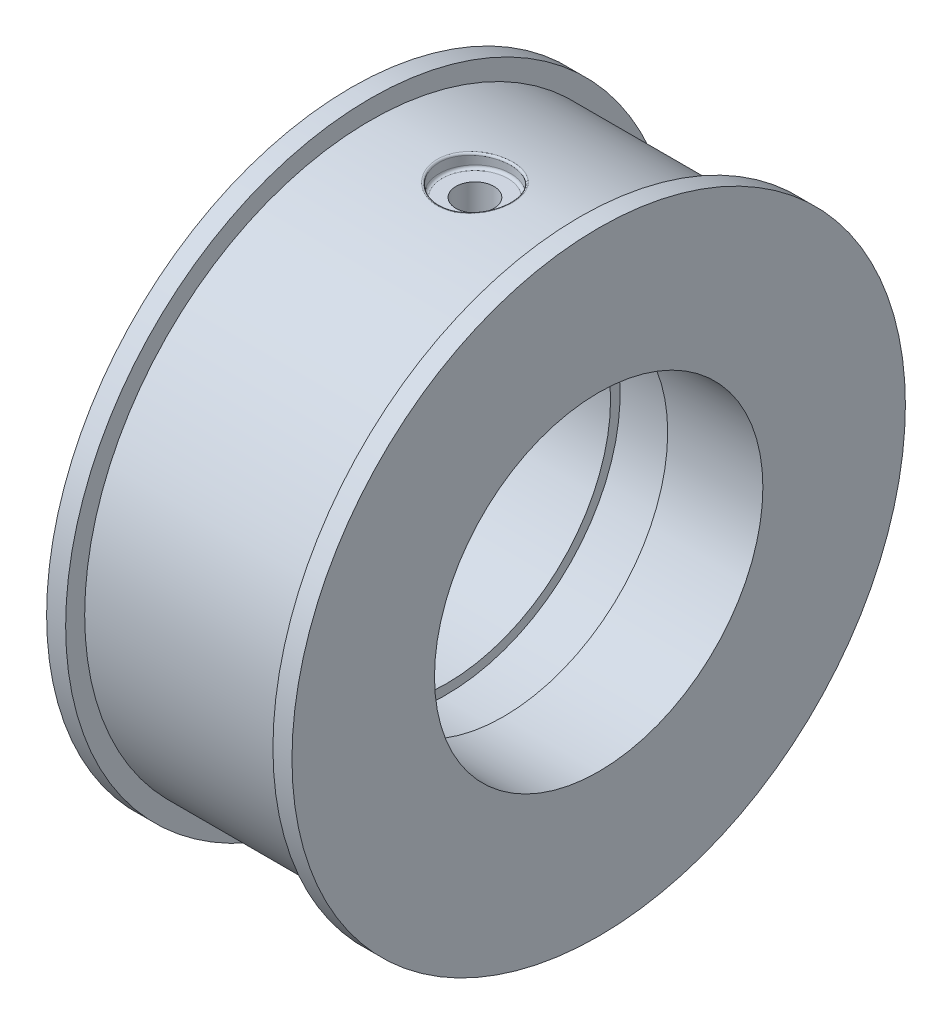
from build123d import *

# Parameters (mm, degrees)
HOLE1_D           = 7.5
HOLE1_DEPTH       = 1.5
HOLE2_REACH       = 72.963
HOLE2_BORE_R      = 2
DOWEL_HOLE1_D     = 4
DOWEL_HOLE1_DEPTH = 4
DOWEL_HOLE1_TIP   = 1.201721238
FILLET1_R         = 0.2
FILLET2_R         = 0.3


with BuildPart() as part:
    # Sketch1 → Revolve1 (revolve)
    with BuildSketch(Plane.XY, mode=Mode.PRIVATE) as revolve1_sk:
        Polygon((-8.389660143, 17.25), (-8.389660143, 32), (-6.389660143, 32), (-6.389660143, 30), (15.610339857, 30), (15.610339857, 32.223034735), (17.610339857, 32.223034735), (17.610339857, 17.25), (7.610339857, 17.25), (7.610339857, 18.25), (1.610339857, 18.25), (1.610339857, 17.25), align=None)
    revolve(revolve1_sk.sketch.rotate(Axis((-19.036826505, 0, 0), (1, 0, 0)), 90), axis=Axis((-19.036826505, 0, 0), (1, 0, 0)))

    # Hole1
    with Locations(Plane(origin=(0, 30, 0), x_dir=(1, 0, 0), z_dir=(0, 1, 0))):
        with Locations((4.610339857, 0)):
            Hole(HOLE1_D / 2, depth=HOLE1_DEPTH)

    # Hole2 bore → Hole2 (cut, up to next)
    with BuildSketch(Plane(origin=(0, 28.5, 0), x_dir=(1, 0, 0), z_dir=(0, 1, 0)), mode=Mode.PRIVATE) as hole2_sk1:
        with Locations((4.610339857, 0)):
            Circle(HOLE2_BORE_R)
    hole2_tool1 = extrude(hole2_sk1.sketch, amount=-HOLE2_REACH, mode=Mode.PRIVATE) & part.part
    add(hole2_tool1.solids().sort_by_distance((4.61034, 28.5, 0))[0], mode=Mode.SUBTRACT)

    # Dowel Hole1
    with Locations(Plane(origin=(0, -30, 0), x_dir=(-1, 0, 0), z_dir=(0, -1, 0))):
        with Locations((-4.610339857, 0)):
            Hole(DOWEL_HOLE1_D / 2, depth=DOWEL_HOLE1_DEPTH)
            with Locations((0, 0, -(DOWEL_HOLE1_DEPTH + DOWEL_HOLE1_TIP / 2))):  # 118° drill point
                Cone(0, DOWEL_HOLE1_D / 2, DOWEL_HOLE1_TIP, mode=Mode.SUBTRACT)

    # Fillet1
    fillet1_edges = [part.edges().sort_by_distance(p)[0] for p in [
        (8.360339864, 29.999999997, -1e-09),
    ]]
    fillet(fillet1_edges, radius=FILLET1_R)

    # Fillet2
    fillet2_edges = [part.edges().sort_by_distance(p)[0] for p in [
        (8.360339857, 28.5, 0),
    ]]
    fillet(fillet2_edges, radius=FILLET2_R)


solid = part.part
